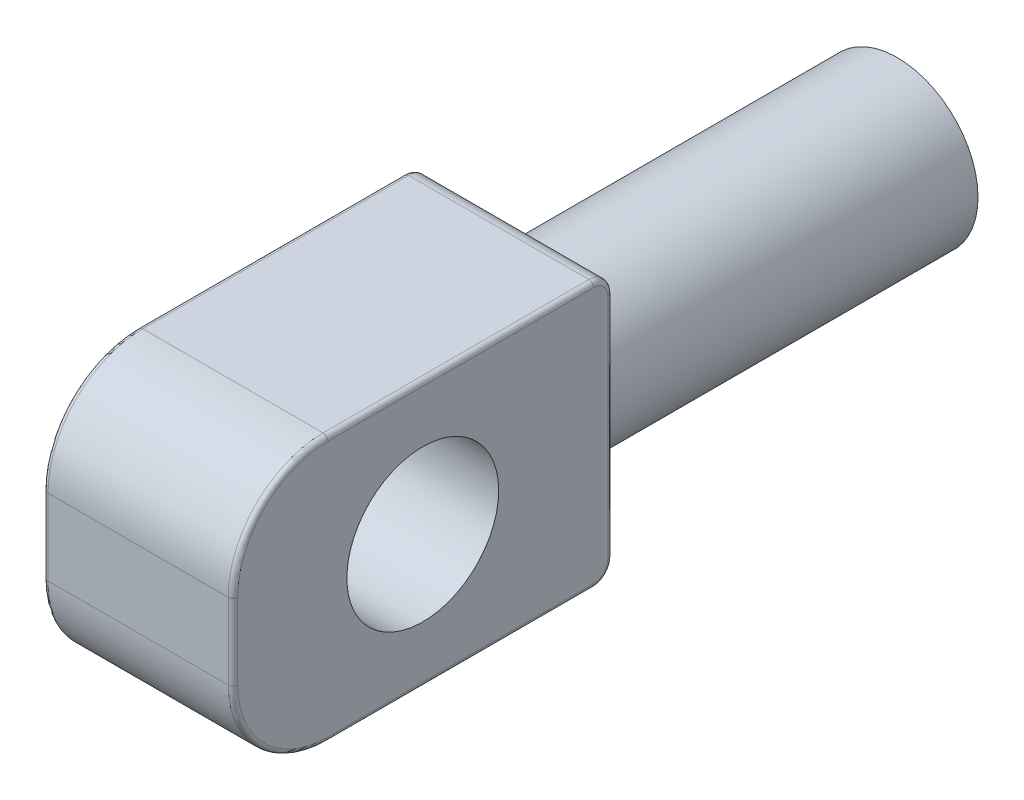
from build123d import *

# Parameters (mm, degrees)
SKETCH1_R           = 4.25
BOSS_EXTRUDE1_DEPTH = 20
BOSS_EXTRUDE2_DEPTH = 5
FILLET1_R           = 0.25
SKETCH5_R           = 4
CUT_EXTRUDE1_DEPTH  = 10


with BuildPart() as part:
    # Sketch1 → Boss-Extrude1 (new body)
    with BuildSketch(Plane.XY):
        Circle(SKETCH1_R)
    extrude(amount=BOSS_EXTRUDE1_DEPTH)

    # Sketch4 → M3.5 Tapped Hole1 (revolve, cut)
    with BuildSketch(Plane.YZ):
        Polygon((0, 0), (0, 10.871247898), (1.45, 10), (1.45, 0.325), (1.775, 0), align=None)
    revolve(axis=Axis((0, 0, -6.35), (0, 0, 1)), mode=Mode.SUBTRACT)


with BuildPart() as body_2:
    # Sketch2 → Boss-Extrude2 (new, symmetric)
    with BuildSketch(Plane(origin=(0, 0, 0), x_dir=(0, 0, -1), z_dir=(1, 0, 0))):
        with BuildLine():
            Line((-21.004909906, -7), (-35.004909906, -7))
            ThreePointArc((-35.004909906, -7), (-38.540443812, -5.535533906), (-40.004909906, -2))
            Line((-40.004909906, -2), (-40.004909906, 2))
            ThreePointArc((-40.004909906, 2), (-38.540443812, 5.535533906), (-35.004909906, 7))
            Line((-35.004909906, 7), (-21.004909906, 7))
            ThreePointArc((-21.004909906, 7), (-20.297803125, 6.707106781), (-20.004909906, 6))
            Line((-20.004909906, 6), (-20.004909906, -6))
            ThreePointArc((-20.004909906, -6), (-20.297803125, -6.707106781), (-21.004909906, -7))
        make_face()
    extrude(amount=BOSS_EXTRUDE2_DEPTH, both=True)

    # Fillet1
    fillet1_edges = [body_2.edges().sort_by_distance(p)[0] for p in [
        (-5, 0, 20.004909906),
        (-5, -6.707106781, 20.297803125),
        (-5, -7, 28.004909906),
        (-5, -5.535533906, 38.540443812),
        (5, -6.707106781, 20.297803125),
        (5, 0, 20.004909906),
        (5, 6.707106781, 20.297803125),
        (5, 7, 28.004909906),
        (5, 5.535533906, 38.540443812),
        (5, 0, 40.004909906),
        (5, -5.535533906, 38.540443812),
        (-5, 0, 40.004909906),
        (5, -7, 28.004909906),
        (-5, 5.535533906, 38.540443812),
        (-5, 7, 28.004909906),
        (-5, 6.707106781, 20.297803125),
    ]]
    fillet(fillet1_edges, radius=FILLET1_R)

    # Sketch5 → Cut-Extrude1 (cut)
    with BuildSketch(Plane(origin=(5, 0, 0), x_dir=(0, 0, -1), z_dir=(1, 0, 0))):
        with Locations((-30.004909906, 0)):
            Circle(SKETCH5_R)
    extrude(amount=-CUT_EXTRUDE1_DEPTH, mode=Mode.SUBTRACT)


solid = Compound([part.part, body_2.part])
